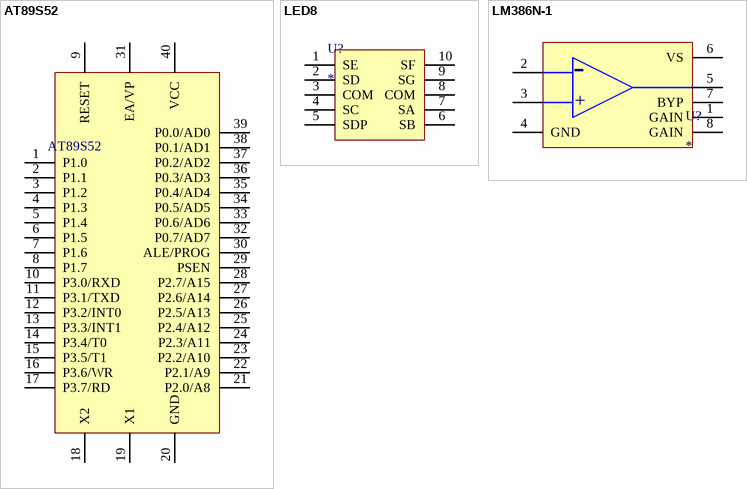
[diagram p0: symbols AT89S52 to LM386N-1]
# Altium schematic symbol library MISC82805-7.SchLib: 3 symbols
Pins are listed as number, name and electrical type; pins without a type are passive.


## AT89S52
designator AT89S52
footprint AT89S52
pins: 1 P1.0, 2 P1.1, 3 P1.2, 4 P1.3, 5 P1.4, 6 P1.5, 7 P1.6, 8 P1.7, 9 RESET, 10 P3.0/RXD, 11 P3.1/TXD, 12 P3.2/INT0, 13 P3.3/INT1, 14 P3.4/T0, 15 P3.5/T1, 16 P3.6/WR, 17 P3.7/RD, 18 X2, 19 X1, 20 GND, 21 P2.0/A8, 22 P2.1/A9, 23 P2.2/A10, 24 P2.3/A11, 25 P2.4/A12, 26 P2.5/A13, 27 P2.6/A14, 28 P2.7/A15, 29 PSEN, 30 ALE/PROG, 31 EA/VP, 32 P0.7/AD7, 33 P0.6/AD6, 34 P0.5/AD5, 35 P0.4/AD4, 36 P0.3/AD3, 37 P0.2/AD2, 38 P0.1/AD1, 39 P0.0/AD0, 40 VCC

## LED8
designator U?
footprint LED8
pins: 1 SE, 2 SD, 3 COM, 4 SC, 5 SDP, 6 SB, 7 SA, 8 COM, 9 SG, 10 SF

## LM386N-1
designator U?
footprint LM386N-1
pins: 1 GAIN, 2 GAIN, 3 GAIN, 4 GND, 5 GND, 6 VS, 7 BYP, 8 GAIN